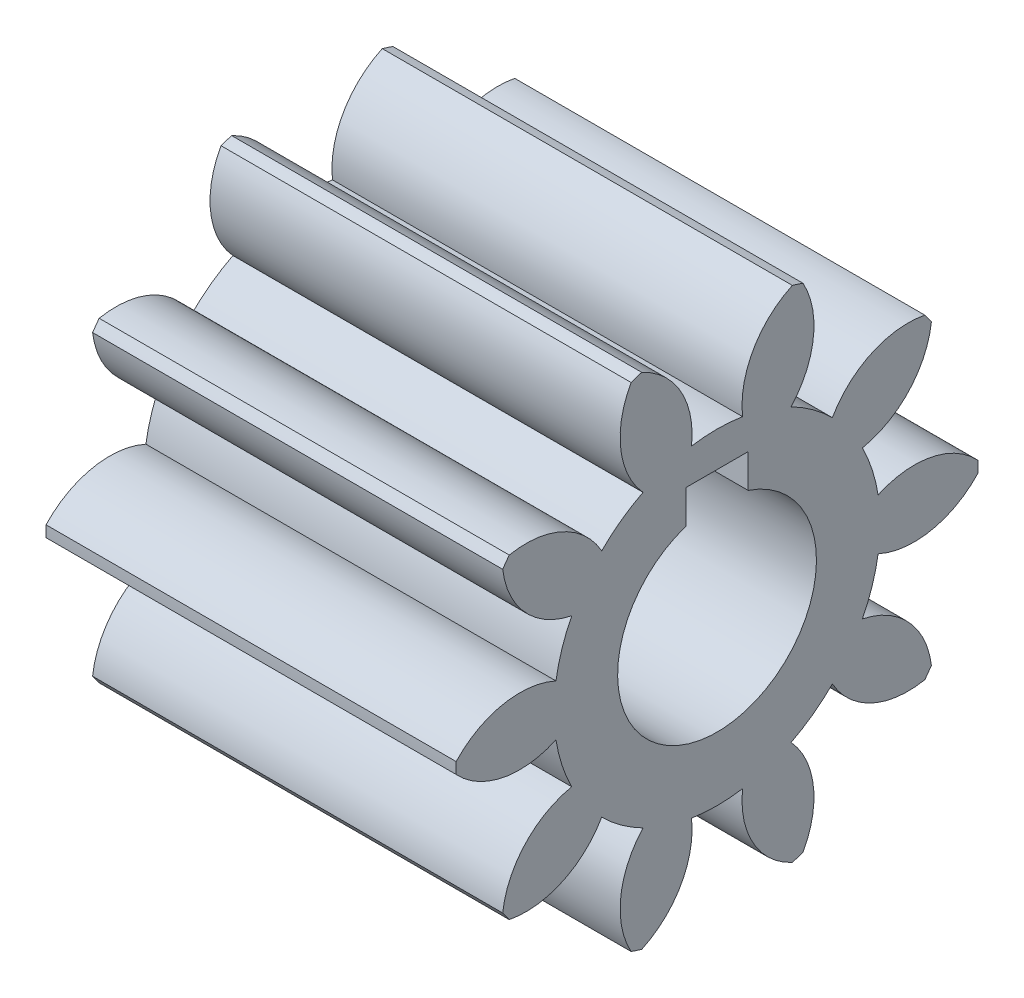
from build123d import *

# Parameters (mm, degrees)
BOSS_EXTRUDE1_DEPTH = 33


with BuildPart() as part:
    # Sketch1 → Boss-Extrude1 (new body)
    with BuildSketch(Plane(origin=(33, 0, 0), x_dir=(0, 0, -1), z_dir=(1, 0, 0))):
        with BuildLine():
            ThreePointArc((20.995176507, 0.450070465), (17.237696927, 2.548883943), (12.962492698, 2.05259812))
            ThreePointArc((12.962492698, 2.05259812), (12.48166572, 4.055539034), (11.693363786, 5.958575279))
            ThreePointArc((11.693363786, 5.958575279), (15.443786149, 8.06997361), (17.249999376, 11.976540465))
            ThreePointArc((17.249999376, 11.976540465), (16.989356882, 12.343490298), (16.720909812, 12.704769776))
            ThreePointArc((16.720909812, 12.704769776), (12.447393366, 12.194154464), (9.280389979, 9.279748803))
            ThreePointArc((9.280389979, 9.279748803), (7.714093651, 10.617539034), (5.957767351, 11.693775447))
            ThreePointArc((5.957767351, 11.693775447), (7.750873978, 15.606375533), (6.91590879, 19.828520006))
            ThreePointArc((6.91590879, 19.828520006), (6.489356882, 19.972186842), (6.059823892, 20.106678851))
            ThreePointArc((6.059823892, 20.106678851), (2.902608611, 17.181672443), (2.053493716, 12.96235085))
            ThreePointArc((2.053493716, 12.96235085), (0, 13.124), (-2.053493716, 12.96235085))
            ThreePointArc((-2.053493716, 12.96235085), (-2.902608611, 17.181672443), (-6.059823892, 20.106678851))
            ThreePointArc((-6.059823892, 20.106678851), (-6.489356882, 19.972186842), (-6.91590879, 19.828520006))
            ThreePointArc((-6.91590879, 19.828520006), (-7.750873978, 15.606375533), (-5.957767351, 11.693775447))
            ThreePointArc((-5.957767351, 11.693775447), (-7.714093651, 10.617539034), (-9.280389979, 9.279748803))
            ThreePointArc((-9.280389979, 9.279748803), (-12.447393366, 12.194154464), (-16.720909812, 12.704769776))
            ThreePointArc((-16.720909812, 12.704769776), (-16.989356882, 12.343490298), (-17.249999376, 11.976540465))
            ThreePointArc((-17.249999376, 11.976540465), (-15.443786149, 8.06997361), (-11.693363786, 5.958575279))
            ThreePointArc((-11.693363786, 5.958575279), (-12.48166572, 4.055539034), (-12.962492698, 2.05259812))
            ThreePointArc((-12.962492698, 2.05259812), (-17.237696927, 2.548883943), (-20.995176507, 0.450070465))
            ThreePointArc((-20.995176507, 0.450070465), (-21, 0), (-20.995176507, -0.450070465))
            ThreePointArc((-20.995176507, -0.450070465), (-17.237696927, -2.548883943), (-12.962492698, -2.05259812))
            ThreePointArc((-12.962492698, -2.05259812), (-12.48166572, -4.055539034), (-11.693363786, -5.958575279))
            ThreePointArc((-11.693363786, -5.958575279), (-15.443786149, -8.06997361), (-17.249999376, -11.976540465))
            ThreePointArc((-17.249999376, -11.976540465), (-16.989356882, -12.343490298), (-16.720909812, -12.704769776))
            ThreePointArc((-16.720909812, -12.704769776), (-12.447393366, -12.194154464), (-9.280389979, -9.279748803))
            ThreePointArc((-9.280389979, -9.279748803), (-7.714093651, -10.617539034), (-5.957767351, -11.693775447))
            ThreePointArc((-5.957767351, -11.693775447), (-7.750873978, -15.606375533), (-6.91590879, -19.828520006))
            ThreePointArc((-6.91590879, -19.828520006), (-6.489356882, -19.972186842), (-6.059823892, -20.106678851))
            ThreePointArc((-6.059823892, -20.106678851), (-2.902608611, -17.181672443), (-2.053493716, -12.96235085))
            ThreePointArc((-2.053493716, -12.96235085), (0, -13.124), (2.053493716, -12.96235085))
            ThreePointArc((2.053493716, -12.96235085), (2.902608611, -17.181672443), (6.059823892, -20.106678851))
            ThreePointArc((6.059823892, -20.106678851), (6.489356882, -19.972186842), (6.91590879, -19.828520006))
            ThreePointArc((6.91590879, -19.828520006), (7.750873978, -15.606375533), (5.957767351, -11.693775447))
            ThreePointArc((5.957767351, -11.693775447), (7.714093651, -10.617539034), (9.280389979, -9.279748803))
            ThreePointArc((9.280389979, -9.279748803), (12.447393366, -12.194154464), (16.720909812, -12.704769776))
            ThreePointArc((16.720909812, -12.704769776), (16.989356882, -12.343490298), (17.249999376, -11.976540465))
            ThreePointArc((17.249999376, -11.976540465), (15.443786149, -8.06997361), (11.693363786, -5.958575279))
            ThreePointArc((11.693363786, -5.958575279), (12.48166572, -4.055539034), (12.962492698, -2.05259812))
            ThreePointArc((12.962492698, -2.05259812), (17.237696927, -2.548883943), (20.995176507, -0.450070465))
            ThreePointArc((20.995176507, -0.450070465), (21, 0), (20.995176507, 0.450070465))
        make_face()
        with BuildLine():
            Line((2.5, 10.3), (2.5, 7.599342077))
            ThreePointArc((2.5, 7.599342077), (0, -8), (-2.5, 7.599342077))
            Line((-2.5, 7.599342077), (-2.5, 10.3))
            Line((-2.5, 10.3), (2.5, 10.3))
        make_face(mode=Mode.SUBTRACT)
    extrude(amount=-BOSS_EXTRUDE1_DEPTH)


solid = part.part
